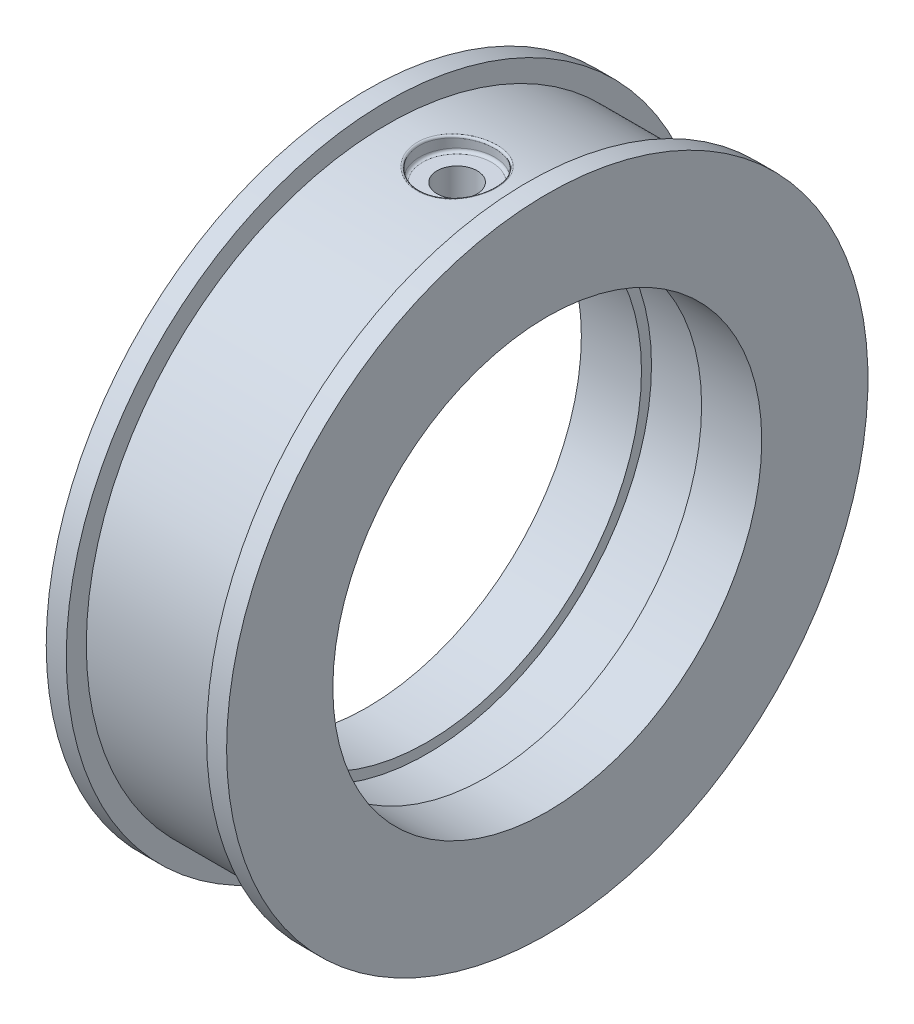
from build123d import *

# Parameters (mm, degrees)
HOLE1_D           = 7.5
HOLE1_DEPTH       = 1.5
HOLE2_REACH       = 71.113
HOLE2_BORE_R      = 2
DOWEL_HOLE1_D     = 4
DOWEL_HOLE1_DEPTH = 4
DOWEL_HOLE1_TIP   = 1.201721238
FILLET1_R         = 0.2
FILLET2_R         = 0.3


with BuildPart() as part:
    # Sketch1 → Revolve1 (revolve)
    with BuildSketch(Plane.XY, mode=Mode.PRIVATE) as revolve1_sk:
        Polygon((-8.389660143, 21.4), (-8.389660143, 32), (-6.389660143, 32), (-6.389660143, 30), (7.610339857, 30), (7.610339857, 32), (9.610339857, 32), (9.610339857, 21.4), (3.610339857, 21.4), (3.610339857, 22.4), (-2.389660143, 22.4), (-2.389660143, 21.4), align=None)
    revolve(revolve1_sk.sketch.rotate(Axis((-19.036826505, 0, 0), (1, 0, 0)), 90), axis=Axis((-19.036826505, 0, 0), (1, 0, 0)))

    # Hole1
    with Locations(Plane(origin=(0, 30, 0), x_dir=(1, 0, 0), z_dir=(0, 1, 0))):
        with Locations((0.610339857, 0)):
            Hole(HOLE1_D / 2, depth=HOLE1_DEPTH)

    # Hole2 bore → Hole2 (cut, up to next)
    with BuildSketch(Plane(origin=(0, 28.5, 0), x_dir=(1, 0, 0), z_dir=(0, 1, 0)), mode=Mode.PRIVATE) as hole2_sk1:
        with Locations((0.610339857, 0)):
            Circle(HOLE2_BORE_R)
    hole2_tool1 = extrude(hole2_sk1.sketch, amount=-HOLE2_REACH, mode=Mode.PRIVATE) & part.part
    add(hole2_tool1.solids().sort_by_distance((0.61034, 28.5, 0))[0], mode=Mode.SUBTRACT)

    # Dowel Hole1
    with Locations(Plane(origin=(0, -30, 0), x_dir=(-1, 0, 0), z_dir=(0, -1, 0))):
        with Locations((-0.610339857, 0)):
            Hole(DOWEL_HOLE1_D / 2, depth=DOWEL_HOLE1_DEPTH)
            with Locations((0, 0, -(DOWEL_HOLE1_DEPTH + DOWEL_HOLE1_TIP / 2))):  # 118° drill point
                Cone(0, DOWEL_HOLE1_D / 2, DOWEL_HOLE1_TIP, mode=Mode.SUBTRACT)

    # Fillet1
    fillet1_edges = [part.edges().sort_by_distance(p)[0] for p in [
        (4.360339864, 29.999999997, -1e-09),
    ]]
    fillet(fillet1_edges, radius=FILLET1_R)

    # Fillet2
    fillet2_edges = [part.edges().sort_by_distance(p)[0] for p in [
        (4.360339857, 28.5, 0),
    ]]
    fillet(fillet2_edges, radius=FILLET2_R)


solid = part.part
